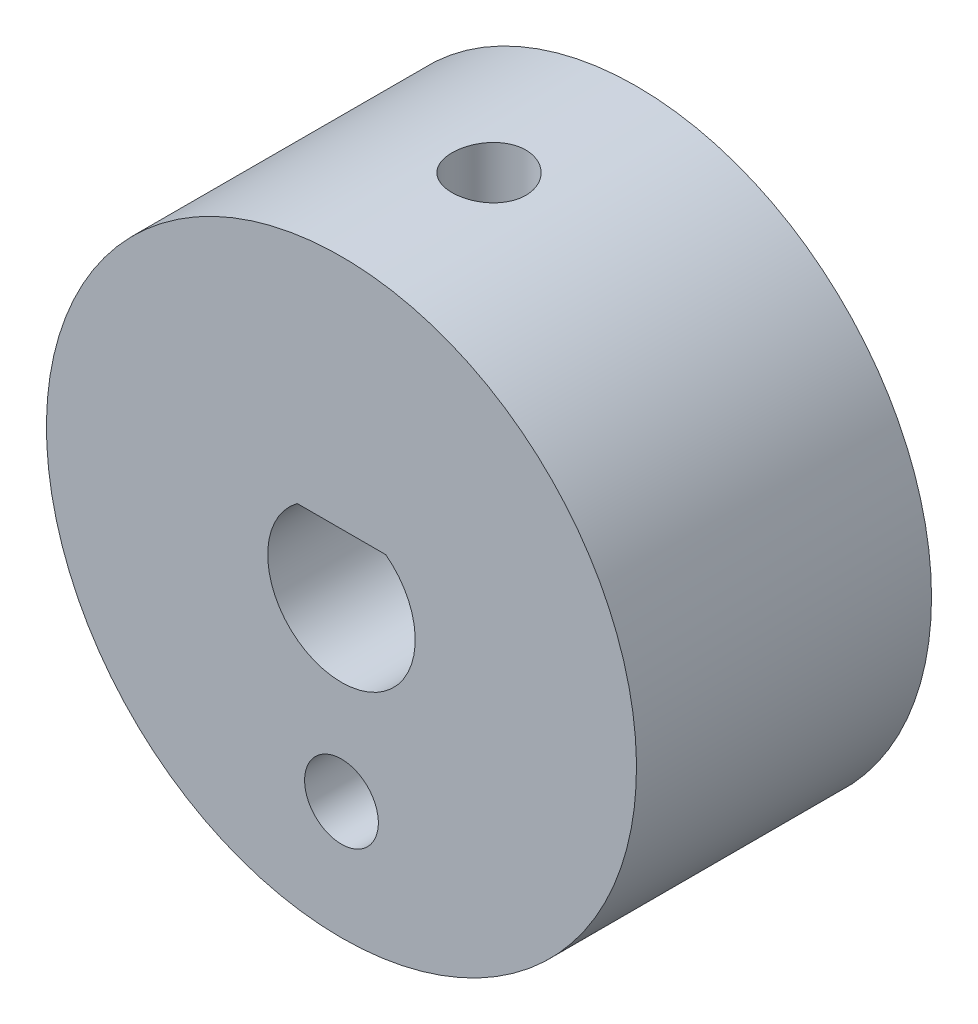
from build123d import *

# Parameters (mm, degrees)
SKETCH_1_R             = 10
EXTRUDE_1_DEPTH        = 10
SKETCH_2_R             = 0.5
CUT_EXTRUDE_1_DEPTH    = 18.320508076
HOLE_WIZARD_M3_1_D     = 2.5
HOLE_WIZARD_M3_1_DEPTH = 8
HOLE_WIZARD_M3_2_D     = 2.5


with BuildPart() as part:
    # 草图1 → 凸台-拉伸1 (new body)
    with BuildSketch(Plane.XY):
        with Locations(Location((0, 0, 0), (0, 0, 270))):
            Circle(SKETCH_1_R)
        with BuildLine():
            Line((-1.5, 2), (1.5, 2))
            ThreePointArc((1.5, 2), (0, -2.5), (-1.5, 2))
        make_face(mode=Mode.SUBTRACT)
    extrude(amount=EXTRUDE_1_DEPTH)

    # 草图2 → 切除-拉伸1 (cut, through all)
    with BuildSketch(Plane.XY.offset(10)):
        with Locations((0, -6)):
            Circle(SKETCH_2_R)
    extrude(amount=-CUT_EXTRUDE_1_DEPTH, mode=Mode.SUBTRACT)

    # M3 螺纹孔1
    with Locations(Plane(origin=(234.411749502, 10, 915.569975215), x_dir=(-1, 0, 0), z_dir=(0, 1, 0))):
        with Locations((234.411749502, -910.569975215)):
            Hole(HOLE_WIZARD_M3_1_D / 2, depth=HOLE_WIZARD_M3_1_DEPTH)

    # M3 螺纹孔2 (through all)
    with Locations(Plane(origin=(0, 0, 0), x_dir=(-1, 0, 0), z_dir=(0, 0, -1))):
        with Locations((0, -6)):
            Hole(HOLE_WIZARD_M3_2_D / 2)


solid = part.part
